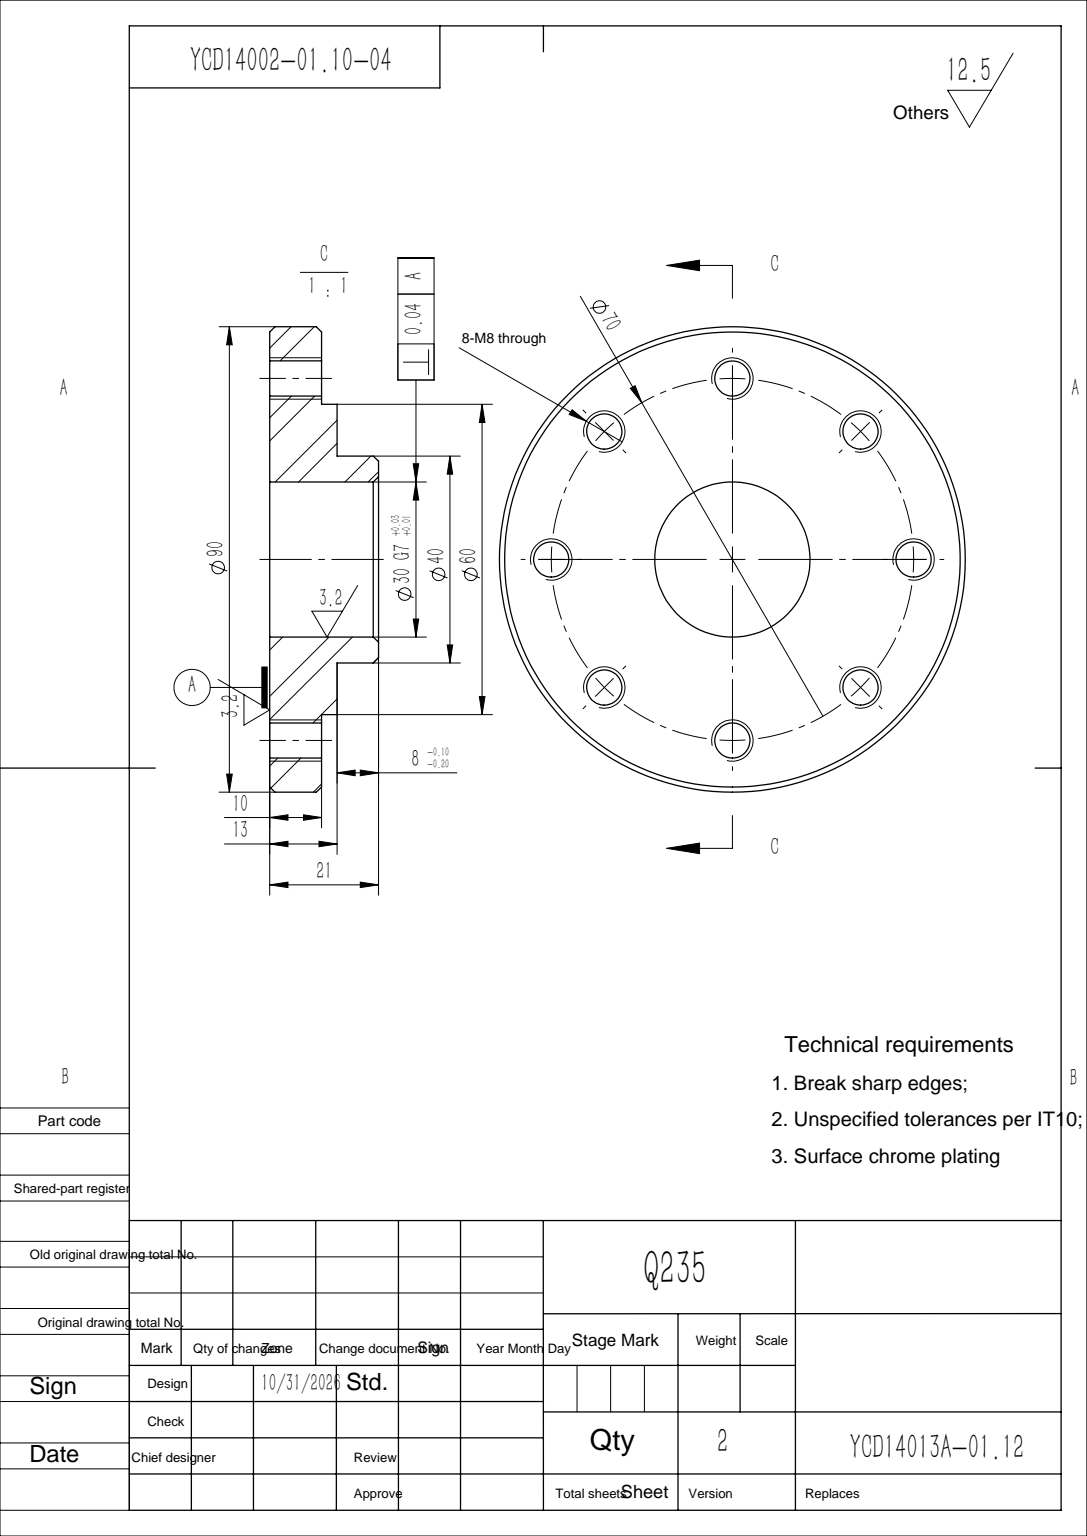
from build123d import *

# Parameters (mm, degrees)
SKETCH1_R           = 20
BOSS_EXTRUDE1_DEPTH = 8
SKETCH3_R           = 30
BOSS_EXTRUDE2_DEPTH = 3
SKETCH4_R           = 45
BOSS_EXTRUDE3_DEPTH = 10
SKETCH5_R           = 15
CUT_EXTRUDE1_DEPTH  = 60
M8_TAPPED_HOLE1_D   = 6.8
CIRPATTERN2_COUNT   = 8
CHAMFER1_SIZE       = 1
CHAMFER2_SIZE       = 1


with BuildPart() as part:
    # Sketch1 → Boss-Extrude1 (new body)
    with BuildSketch(Plane(origin=(0, 0, 0), x_dir=(1, 0, 0), z_dir=(0, 1, 0))):
        with Locations(Location((0, 0, 0), (0, 0, 270))):
            Circle(SKETCH1_R)
    extrude(amount=BOSS_EXTRUDE1_DEPTH)

    # Sketch3 → Boss-Extrude2 (add)
    with BuildSketch(Plane.XZ):
        with Locations(Location((0, 0, 0), (0, 0, 270))):
            Circle(SKETCH3_R)
    extrude(amount=BOSS_EXTRUDE2_DEPTH)

    # Sketch4 → Boss-Extrude3 (add)
    with BuildSketch(Plane.XZ.offset(3)):
        with Locations(Location((0, 0, 0), (0, 0, 270))):
            Circle(SKETCH4_R)
    extrude(amount=BOSS_EXTRUDE3_DEPTH)

    # Sketch5 → Cut-Extrude1 (cut)
    with BuildSketch(Plane(origin=(0, 8, 0), x_dir=(1, 0, 0), z_dir=(0, 1, 0))):
        with Locations(Location((0, 0, 0), (0, 0, 270))):
            Circle(SKETCH5_R)
    extrude(amount=-CUT_EXTRUDE1_DEPTH, mode=Mode.SUBTRACT)

    # M8 Tapped Hole1 (through all)
    with Locations(Plane(origin=(0, -13, 0), x_dir=(-1, 0, 0), z_dir=(0, -1, 0))):
        with Locations((0, -35)):
            m8_tapped_hole1 = Hole(M8_TAPPED_HOLE1_D / 2)

    # CirPattern2: M8 Tapped Hole1 ×8 about axis
    cirpattern2_axis = Axis((0, 0, 0), (0, 1, 0))
    for i in range(1, CIRPATTERN2_COUNT):
        add(m8_tapped_hole1.rotate(cirpattern2_axis, i * 360 / CIRPATTERN2_COUNT), mode=Mode.SUBTRACT)

    # Chamfer1
    chamfer1_edges = [part.edges().sort_by_distance(p)[0] for p in [
        (0, -13, 45),
        (0, -3, 45),
    ]]
    chamfer(chamfer1_edges, length=CHAMFER1_SIZE)

    # Chamfer2
    chamfer2_edges = [part.edges().sort_by_distance(p)[0] for p in [
        (0, 8, -15),
        (0, 8, -20),
    ]]
    chamfer(chamfer2_edges, length=CHAMFER2_SIZE)


solid = part.part
